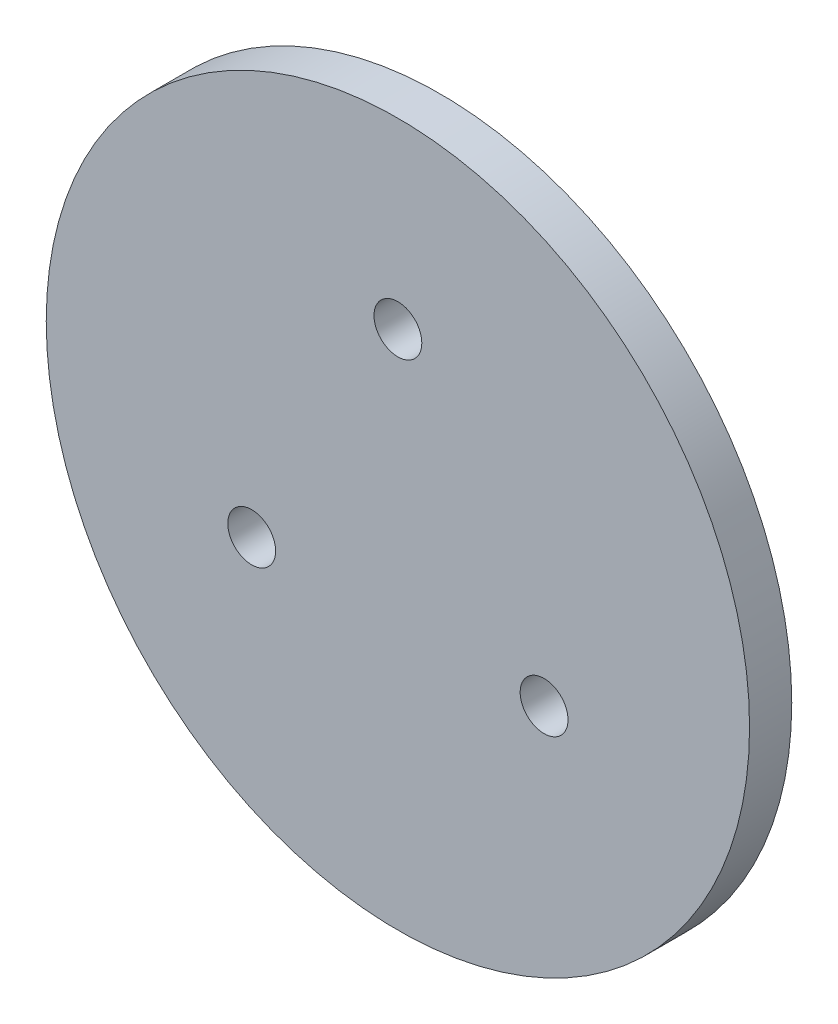
SolidWorks part; units mm, degrees
material "Q235-A"
ref_plane "Front Plane" through (0, 0, 0) normal (0, 0, 1) x (1, 0, 0)
ref_plane "Top Plane" through (0, 0, 0) normal (0, 1, 0) x (1, 0, 0)
ref_plane "Right Plane" through (0, 0, 0) normal (1, 0, 0) x (0, 0, -1)
sketch "Sketch1" plane through (0, 0, 0) normal (0, 0, 1) x (1, 0, 0)
  circle A0 centre (0, 0) radius 125
  circle A1 centre (0, 0) radius 60 construction
  circle A2 centre (0, 60) radius 8.5
  circle A3 centre (0, 0) radius 60 construction
  circle A4 centre (51.9615, -30) radius 8.5
  circle A5 centre (0, 0) radius 60 construction
  circle A6 centre (-51.9615, -30) radius 8.5
  point P18 (0, 0)
  dimension "D1" = 250
  dimension "D2" = 120
  dimension "D3" = 17
  dimension "D4" = 3
extrude "Boss-Extrude1" add sketch "Sketch1" along normal mid plane 15
